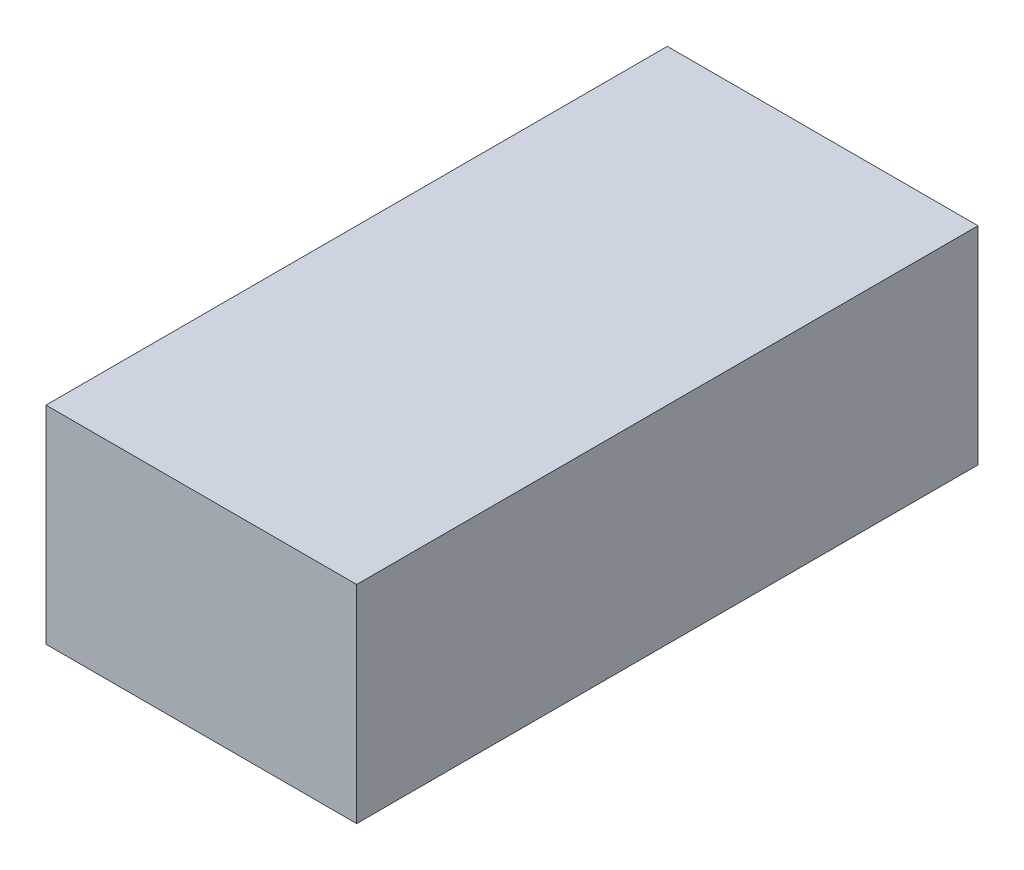
from build123d import *

# Parameters (mm, degrees)
SKETCH1_W           = 150
SKETCH1_H           = 100
BOSS_EXTRUDE1_DEPTH = 300


with BuildPart() as part:
    # Sketch1 → Boss-Extrude1 (new body)
    with BuildSketch(Plane.XY):
        Rectangle(SKETCH1_W, SKETCH1_H)
    extrude(amount=BOSS_EXTRUDE1_DEPTH)


solid = part.part
